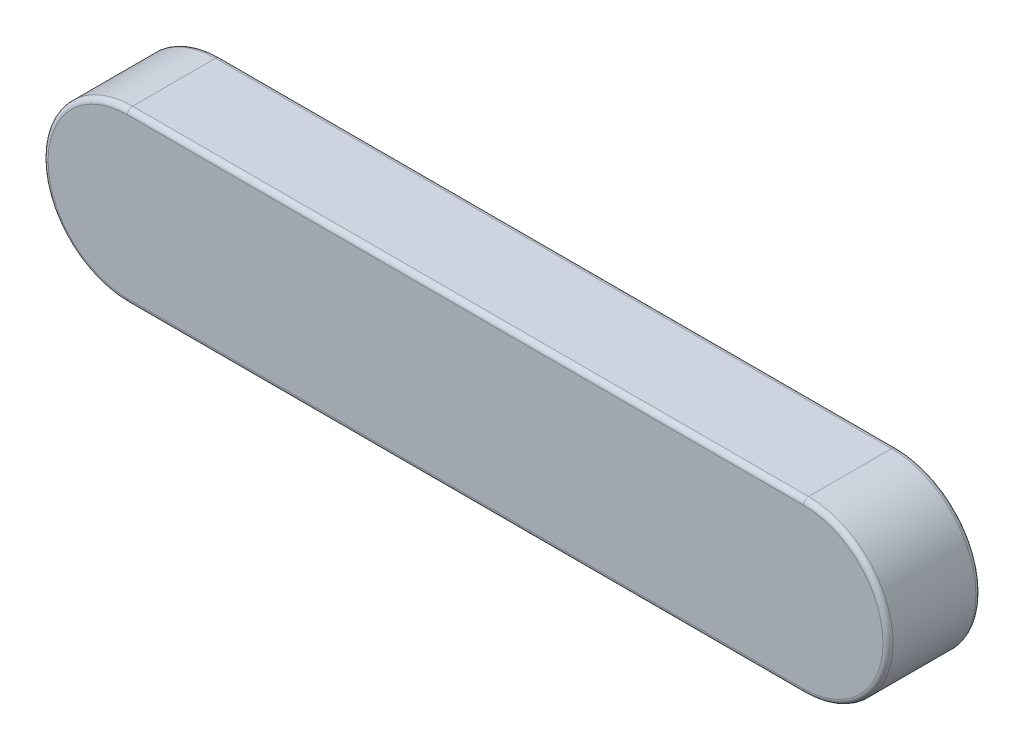
from build123d import *

# Parameters (mm, degrees)
BASE_EXTRUDE_DEPTH = 22
FILLET1_R          = 1.2


with BuildPart() as part:
    # Sketch1 → Base-Extrude (new body)
    with BuildSketch(Plane.XY):
        with BuildLine():
            Line((-80, 20), (80, 20))
            ThreePointArc((80, 20), (100, 0), (80, -20))
            Line((80, -20), (-80, -20))
            ThreePointArc((-80, -20), (-100, 0), (-80, 20))
        make_face()
    extrude(amount=BASE_EXTRUDE_DEPTH)

    # Fillet1
    fillet1_edges = [part.edges().sort_by_distance(p)[0] for p in [
        (100, 0, 22),
        (0, 20, 22),
        (-100, 0, 22),
        (0, 20, 0),
        (100, 0, 0),
        (0, -20, 0),
        (-100, 0, 0),
        (0, -20, 22),
    ]]
    fillet(fillet1_edges, radius=FILLET1_R)


solid = part.part
